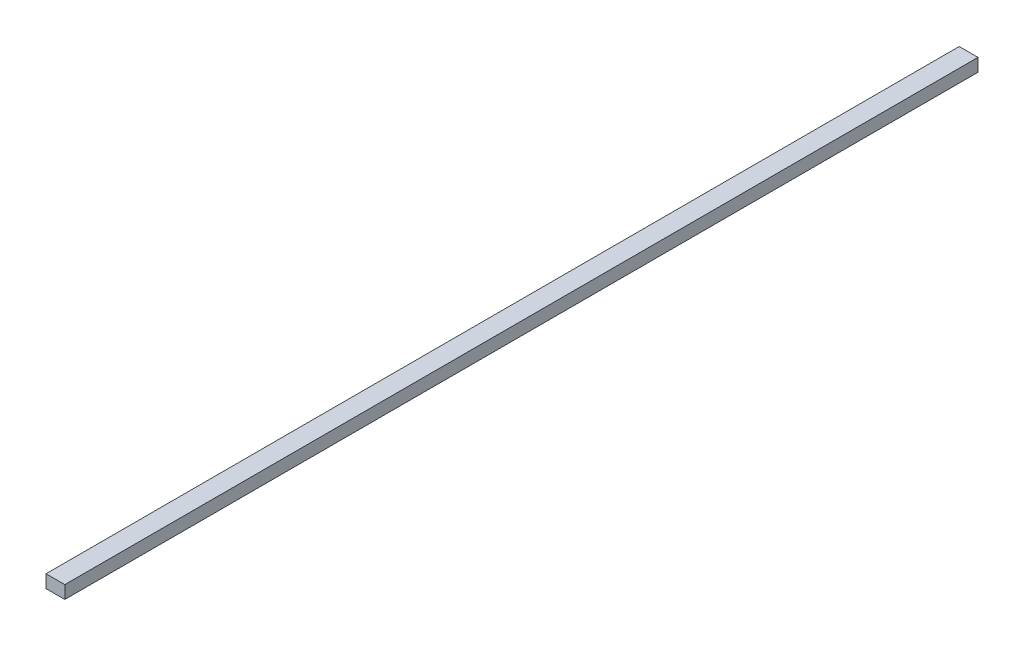
SolidWorks part; units mm, degrees
ref_plane "Front" through (0, 0, 0) normal (0, 0, 1) x (1, 0, 0)
ref_plane "Top" through (0, 0, 0) normal (0, 1, 0) x (1, 0, 0)
ref_plane "Right" through (0, 0, 0) normal (1, 0, 0) x (0, 0, -1)
sketch "Sketch1" plane through (0, 0, 0) normal (0, 0, 1) x (1, 0, 0)
  line L1 (-3.5, 2.6503) -> (3.5, 2.6503)
  line L2 (-3.5, 2.6503) -> (-3.5, -2.1497)
  line L3 (-3.5, -2.1497) -> (3.5, -2.1497)
  line L4 (3.5, 2.6503) -> (3.5, -2.1497)
  dimension "D1" = 7
  dimension "D2" = 4.8
  dimension "D3" = 3.5
extrude "Boss-Extrude1" add sketch "Sketch1" along normal blind 340 contours L1 L4 L3 L2
sketch "Sketch2" plane through (0, 2.6503, 0) normal (0, 1, 0) x (1, 0, 0)
  line L0 (-3.5, -340) -> (3.5, -340) construction
  line L1 (-3.5, -340) -> (-3.5, 0) construction
  circle A0 centre (0, -335) radius 1
  dimension "D2" = 2
  dimension "D1" = 5
  dimension "D3" = 3.5
extrude "Cut-Extrude1" [suppressed] cut sketch "Sketch2" against normal blind 668
sketch "Sketch3" [suppressed] plane through (0, 2.6503, 0) normal (0, 1, 0) x (1, 0, 0)
  circle A0 centre (0, -335) radius 2.5
  dimension "D1" = 5
extrude "Cut-Extrude2" [suppressed] cut sketch "Sketch3" against normal blind 2.5
pattern_linear "LPattern1" [suppressed] count 23 spacing 15
